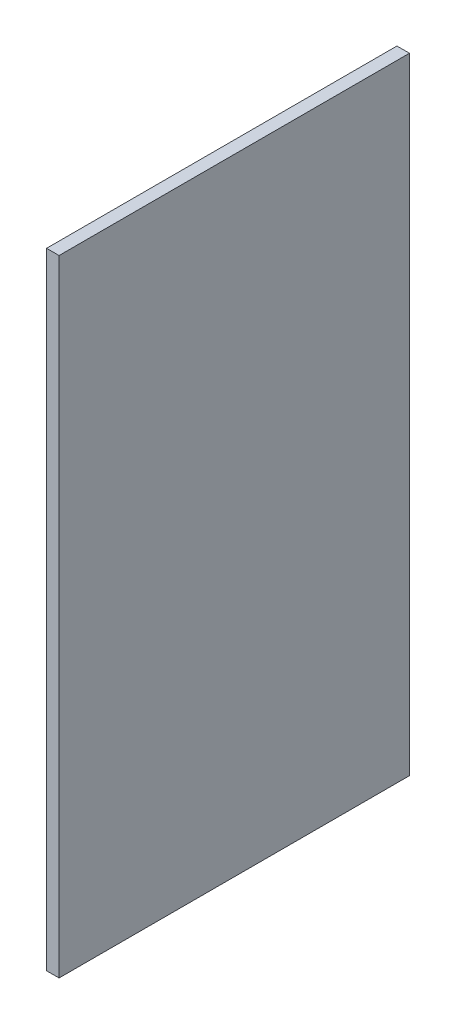
SolidWorks part; units mm, degrees
material "Q235"
ref_plane "前视基准面" through (0, 0, 0) normal (0, 0, 1) x (1, 0, 0)
ref_plane "上视基准面" through (0, 0, 0) normal (0, 1, 0) x (1, 0, 0)
ref_plane "右视基准面" through (0, 0, 0) normal (1, 0, 0) x (0, 0, -1)
sketch "草图1" plane through (0, 0, 0) normal (1, 0, 0) x (0, 0, -1)
  line L1 (0, 0) -> (112, 0)
  line L2 (0, 0) -> (0, 200)
  line L3 (0, 200) -> (112, 200)
  line L4 (112, 0) -> (112, 200)
  dimension "D1" = 112
  dimension "D2" = 200
extrude "凸台-拉伸1" add sketch "草图1" along normal blind 4
